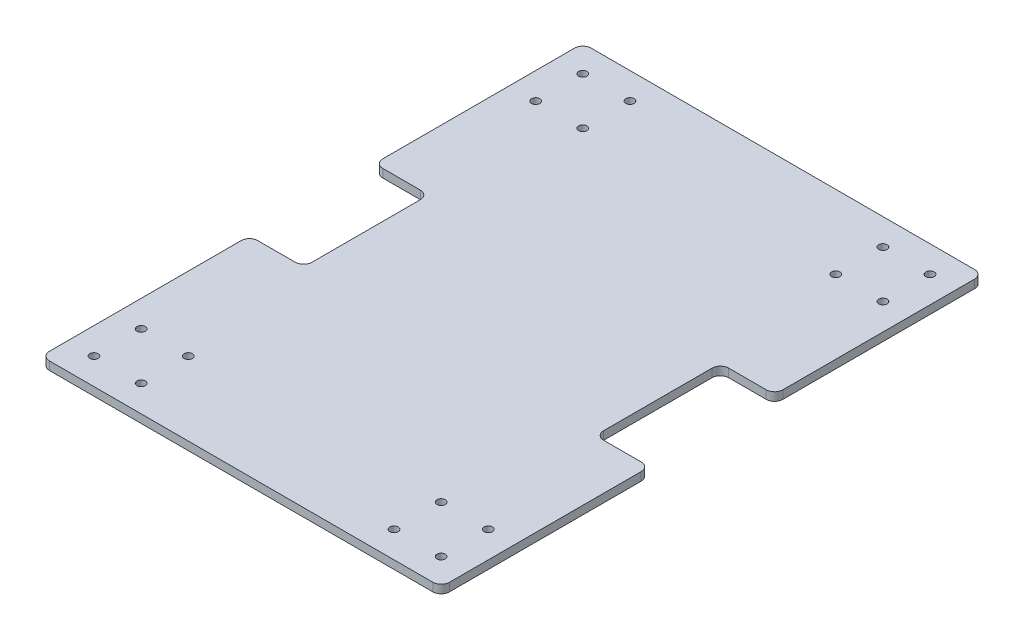
from build123d import *

# Parameters (mm, degrees)
SKETCH1_W           = 480
SKETCH1_H           = 650
BOSS_EXTRUDE1_DEPTH = 10
SKETCH3_W           = 130
SKETCH3_H           = 150
CUT_EXTRUDE1_DEPTH  = 10
FILLET1_R           = 10
FILLET3_R           = 10
SKETCH5_R           = 5
CUT_EXTRUDE2_DEPTH  = 10


with BuildPart() as part:
    # Sketch1 → Boss-Extrude1 (new body)
    with BuildSketch(Plane(origin=(0, 0, 0), x_dir=(1, 0, 0), z_dir=(0, 1, 0))):
        Rectangle(SKETCH1_W, SKETCH1_H)
    extrude(amount=BOSS_EXTRUDE1_DEPTH)

    # Sketch3 → Cut-Extrude1 (cut)
    with BuildSketch(Plane(origin=(0, 10, 0), x_dir=(1, 0, 0), z_dir=(0, 1, 0))):
        with Locations((240, 0)):
            Rectangle(SKETCH3_W, SKETCH3_H)
        with Locations((-240, 0)):
            Rectangle(SKETCH3_W, SKETCH3_H)
    extrude(amount=-CUT_EXTRUDE1_DEPTH, mode=Mode.SUBTRACT)

    # Fillet1
    fillet1_edges = [part.edges().sort_by_distance(p)[0] for p in [
        (240, 5, -75),
        (175, 5, -75),
        (240, 5, 75),
        (175, 5, 75),
        (-240, 5, 75),
        (-175, 5, 75),
        (-175, 5, -75),
        (-240, 5, -75),
    ]]
    fillet(fillet1_edges, radius=FILLET1_R)

    # Fillet3
    fillet3_edges = [part.edges().sort_by_distance(p)[0] for p in [
        (240, 5, 325),
        (-240, 5, 325),
        (-240, 5, -325),
        (240, 5, -325),
    ]]
    fillet(fillet3_edges, radius=FILLET3_R)

    # Sketch5 → Cut-Extrude2 (cut)
    with BuildSketch(Plane(origin=(0, 10, 0), x_dir=(1, 0, 0), z_dir=(0, 1, 0))):
        with Locations(Location((-208.284271247, -293.284271247, 0), (0, 0, 270))):
            Circle(SKETCH5_R)
        with Locations(Location((-208.284271247, -236.715728753, 0), (0, 0, 270))):
            Circle(SKETCH5_R)
        with Locations(Location((-151.715728753, -236.715728753, 0), (0, 0, 270))):
            Circle(SKETCH5_R)
        with Locations(Location((-151.715728753, -293.284271247, 0), (0, 0, 270))):
            Circle(SKETCH5_R)
        with Locations(Location((208.284271247, -293.284271247, 0), (0, 0, 270))):
            Circle(SKETCH5_R)
        with Locations(Location((151.715728753, -293.284271247, 0), (0, 0, 270))):
            Circle(SKETCH5_R)
        with Locations(Location((151.715728753, -236.715728753, 0), (0, 0, 270))):
            Circle(SKETCH5_R)
        with Locations(Location((208.284271247, -236.715728753, 0), (0, 0, 270))):
            Circle(SKETCH5_R)
        with Locations(Location((-208.284271247, 236.715728753, 0), (0, 0, 270))):
            Circle(SKETCH5_R)
        with Locations(Location((208.284271247, 293.284271247, 0), (0, 0, 270))):
            Circle(SKETCH5_R)
        with Locations(Location((208.284271247, 236.715728753, 0), (0, 0, 270))):
            Circle(SKETCH5_R)
        with Locations(Location((151.715728753, 293.284271247, 0), (0, 0, 270))):
            Circle(SKETCH5_R)
        with Locations(Location((151.715728753, 236.715728753, 0), (0, 0, 270))):
            Circle(SKETCH5_R)
        with Locations(Location((-151.715728753, 293.284271247, 0), (0, 0, 270))):
            Circle(SKETCH5_R)
        with Locations(Location((-208.284271247, 293.284271247, 0), (0, 0, 270))):
            Circle(SKETCH5_R)
        with Locations(Location((-151.715728753, 236.715728753, 0), (0, 0, 270))):
            Circle(SKETCH5_R)
    extrude(amount=-CUT_EXTRUDE2_DEPTH, mode=Mode.SUBTRACT)


solid = part.part
